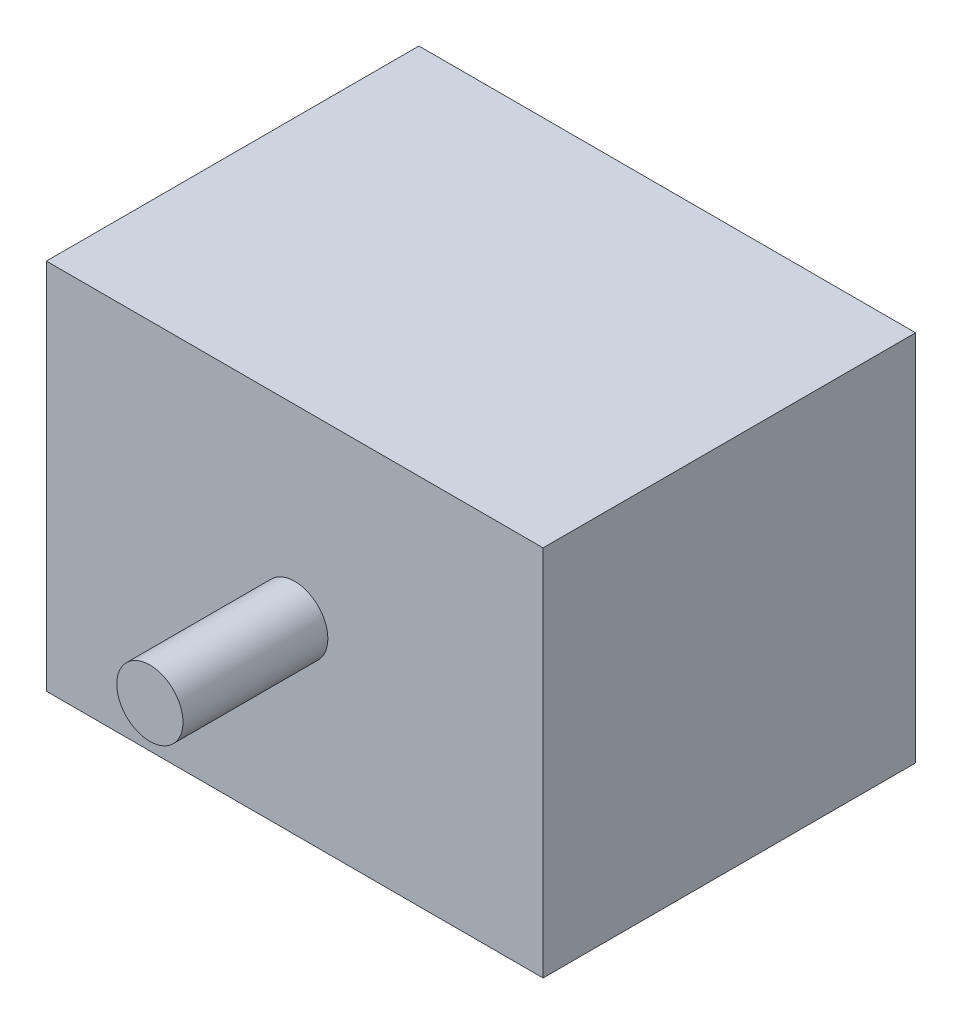
SolidWorks part; units mm, degrees
ref_plane "前视基准面" through (0, 0, 0) normal (0, 0, 1) x (1, 0, 0)
ref_plane "上视基准面" through (0, 0, 0) normal (0, 1, 0) x (1, 0, 0)
ref_plane "右视基准面" through (0, 0, 0) normal (1, 0, 0) x (0, 0, -1)
other "Configuration Table"
sketch "草图1" plane through (0, 0, 0) normal (0, 0, 1) x (1, 0, 0)
  line L0 (-60, -45) -> (60, -45)
  line L1 (60, -45) -> (60, 45)
  line L2 (60, 45) -> (-60, 45)
  line L3 (-60, 45) -> (-60, -45)
  point P0 (0, 0)
  dimension "D1" = 60
  dimension "D2" = 120
  dimension "D3" = 45
  dimension "D4" = 90
extrude "凸台-拉伸1" add sketch "草图1" against normal mid plane 90
sketch "草图2" plane through (0, 0, 0) normal (0, 0, 1) x (1, 0, 0)
  circle A0 centre (0, 0) radius 8
  point P0 (0, 0)
  dimension "D1" = 16
extrude "凸台-拉伸2" add sketch "草图2" against normal mid plane 160
